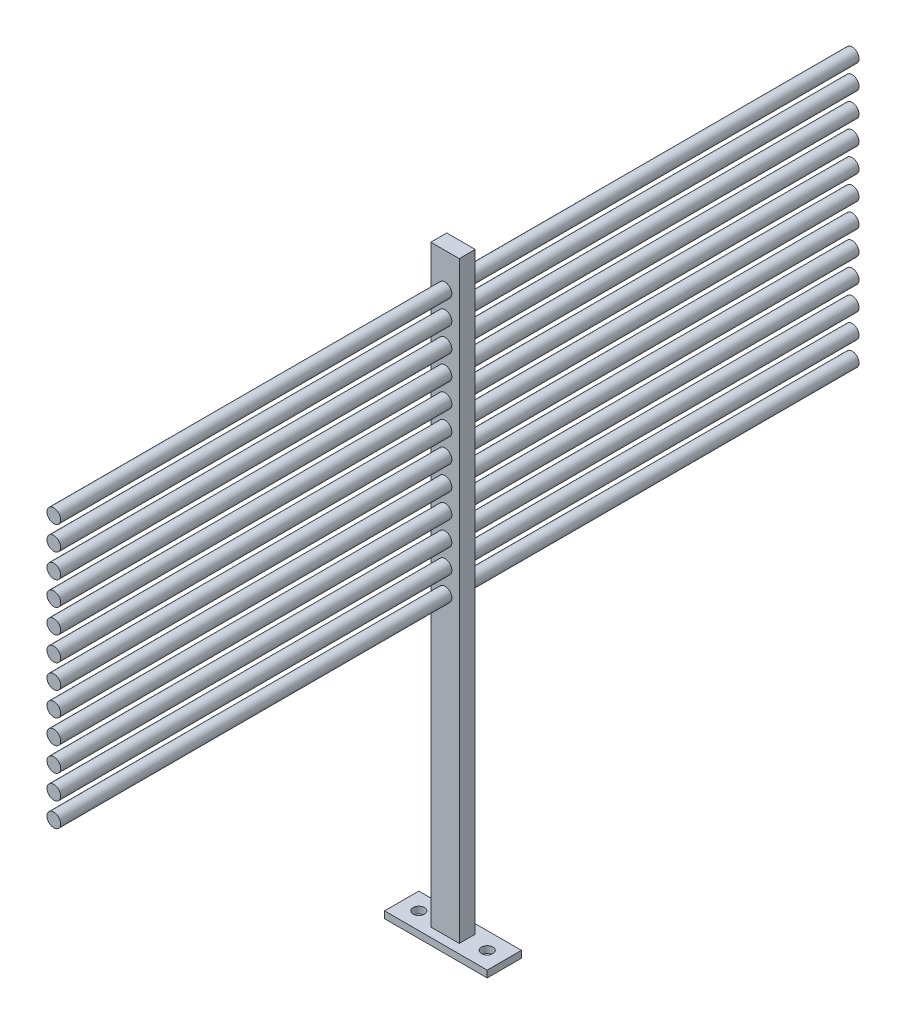
from build123d import *

# Parameters (mm, degrees)
SKETCH1_W                = 25
SKETCH1_H                = 520
BOSS_EXTRUDE1_DEPTH      = 14
BOSS_EXTRUDE2_START      = -7
SKETCH3_R                = 6
BOSS_EXTRUDE2_DEPTH      = 350
LPATTERN1_COUNT          = 12
LPATTERN1_PITCH          = 21
SKETCH4_W                = 90
SKETCH4_H                = 30
BOSS_EXTRUDE3_DEPTH      = 6
M8_CLEARANCE_HOLE1_D     = 10
M8_CLEARANCE_HOLE1_DEPTH = 20
M8_CLEARANCE_HOLE1_TIP   = 3.004303095


with BuildPart() as part:
    # Sketch1 → Boss-Extrude1 (new body)
    with BuildSketch(Plane.XY):
        Rectangle(SKETCH1_W, SKETCH1_H)
    extrude(amount=BOSS_EXTRUDE1_DEPTH)

    # Sketch3 → Boss-Extrude2 (add, symmetric)
    with BuildSketch(Plane.XY.offset(14).offset(BOSS_EXTRUDE2_START)):
        with Locations((0, 230)):
            Circle(SKETCH3_R)
    boss_extrude2 = extrude(amount=BOSS_EXTRUDE2_DEPTH, both=True)

    # LPattern1: Boss-Extrude2 ×12
    with Locations(*[(0, -i * LPATTERN1_PITCH, 0) for i in range(1, LPATTERN1_COUNT)]):
        add(boss_extrude2)

    # Sketch4 → Boss-Extrude3 (add)
    with BuildSketch(Plane.XZ.offset(260)):
        with Locations((0, 7)):
            Rectangle(SKETCH4_W, SKETCH4_H)
    extrude(amount=BOSS_EXTRUDE3_DEPTH)

    # M8 Clearance Hole1
    with Locations(Plane(origin=(0, -260, 0), x_dir=(1, 0, 0), z_dir=(0, 1, 0))):
        with Locations((-30, -7), (30, -7)):
            Hole(M8_CLEARANCE_HOLE1_D / 2, depth=M8_CLEARANCE_HOLE1_DEPTH)
            with Locations((0, 0, -(M8_CLEARANCE_HOLE1_DEPTH + M8_CLEARANCE_HOLE1_TIP / 2))):  # 118° drill point
                Cone(0, M8_CLEARANCE_HOLE1_D / 2, M8_CLEARANCE_HOLE1_TIP, mode=Mode.SUBTRACT)


solid = part.part
